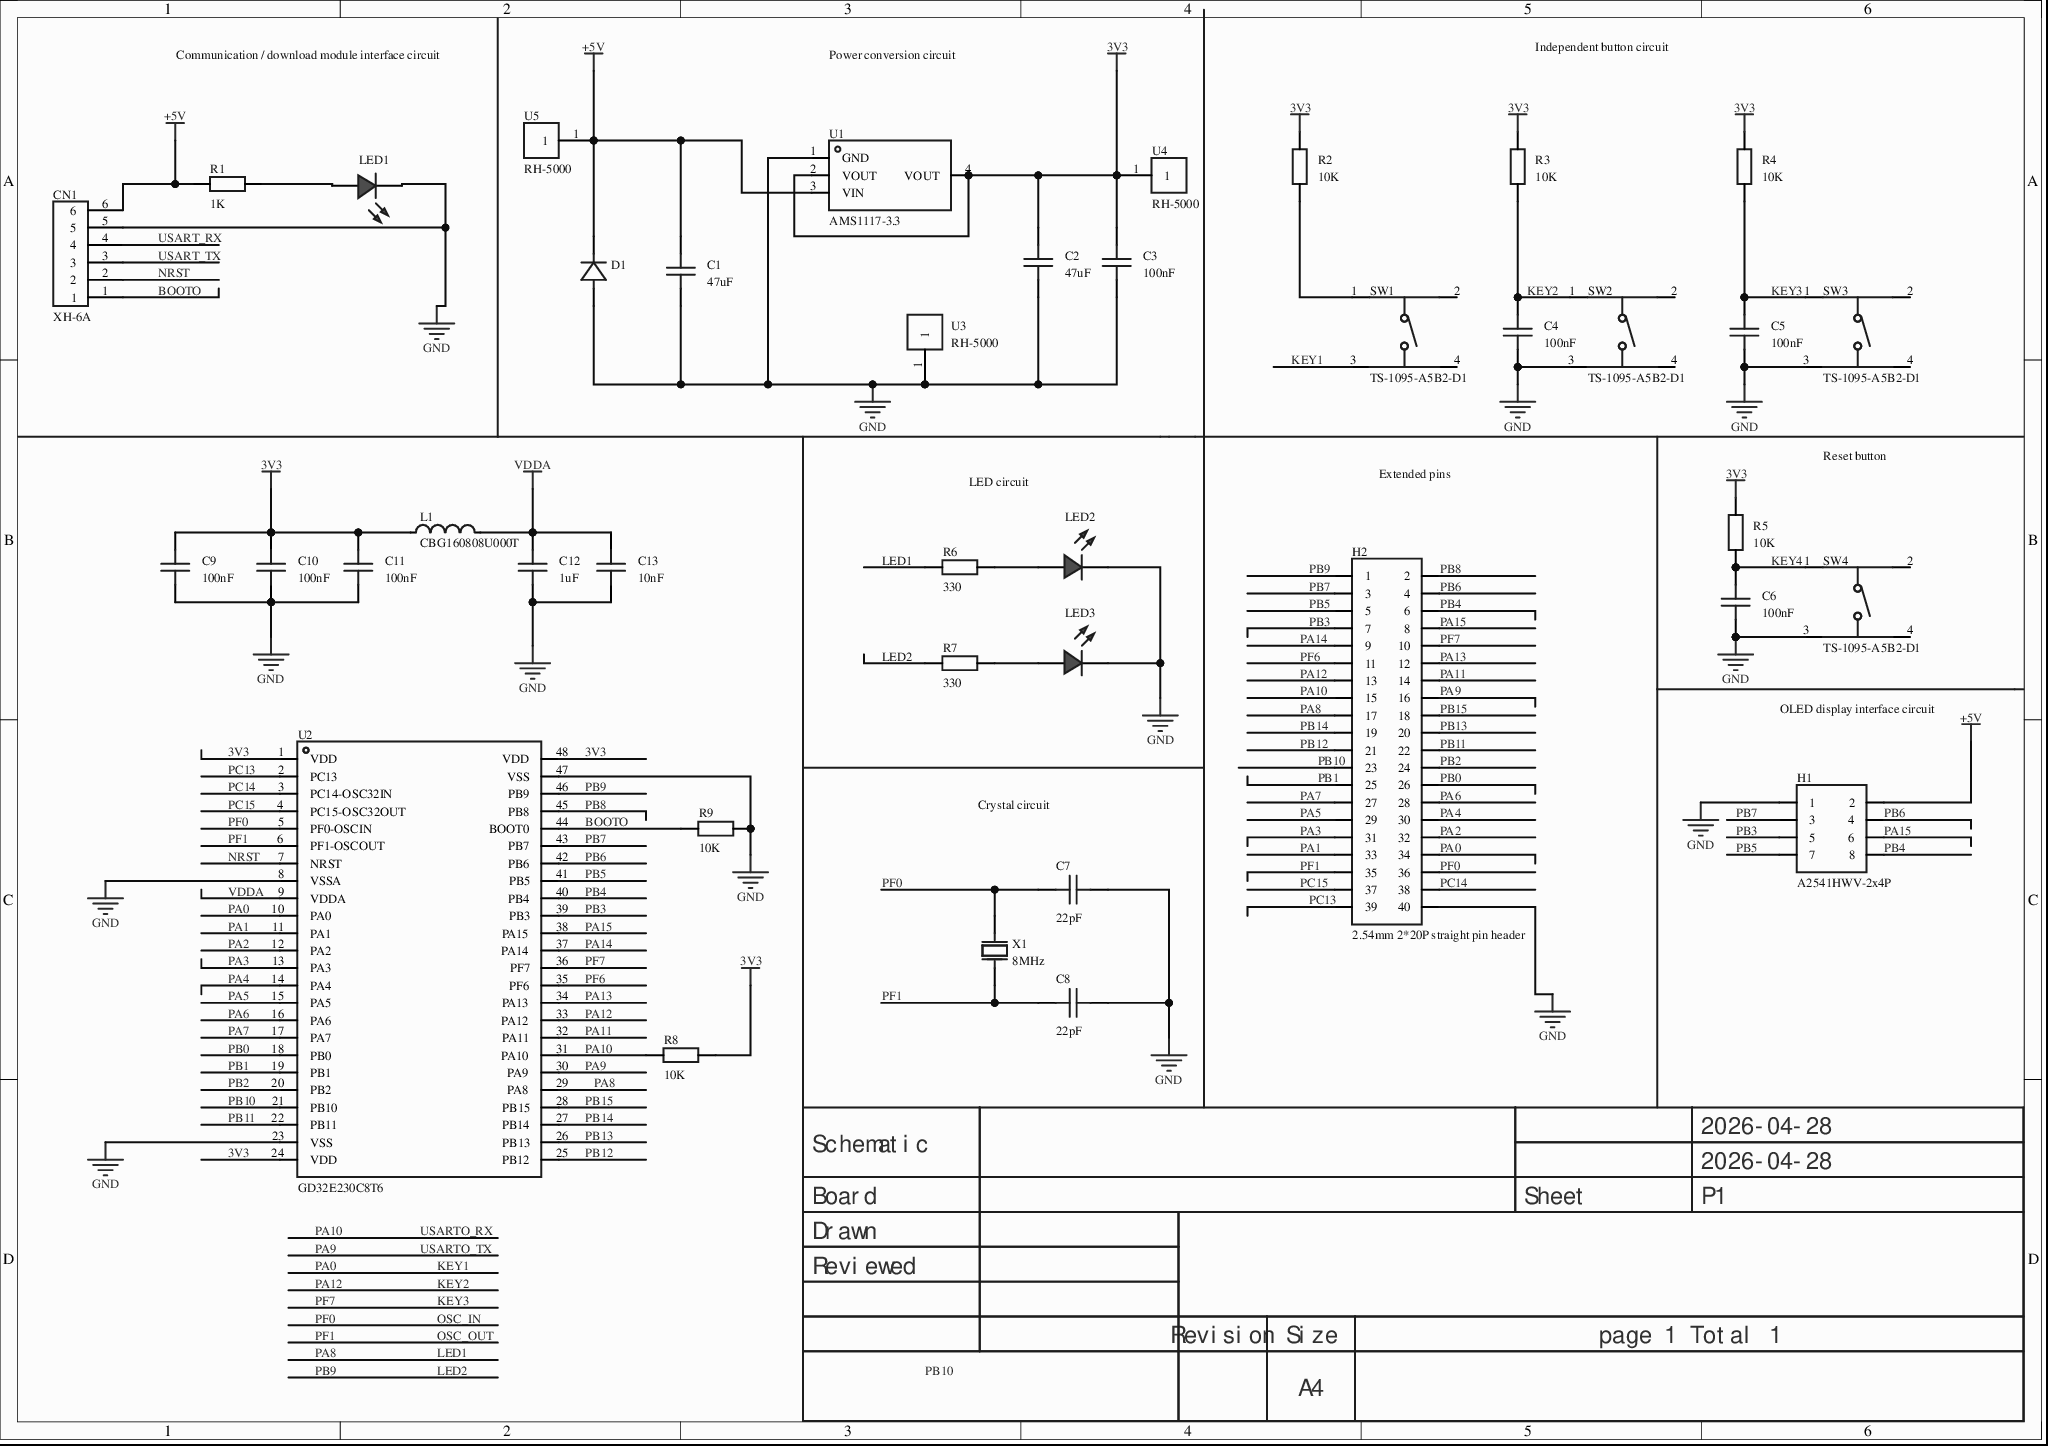
[diagram p0: MISC75379-3.schdoc]
# Altium project MISC75379-2.PrjPcb
1 sheet, 40 parts. Net scope: global (net labels, ports and power ports of the same name join across sheets).
Board file: MISC75379.pcbdoc

## Sheet MISC75379-3.schdoc
size 297 x 209 mm; Version: V1.0; @Project Name: MISC75379; @Update Date: 2026-04-28; @Create Date: 2026-04-28; @Board Name: MISC75379; @Create Time: 14:08:04; @Page Count: 1; @Page No: 1; @Schematic Name: MISC75379; @Update Time: 14:08:04; Size: A4

### Parts
C1  47uF  [C0603]
C2  47uF  [C0603]
C3  100nF  [C0603]
C4  100nF  [C0603]
C5  100nF  [C0603]
C6  100nF  [C0603]
C7  22pF  [C0603]
C8  22pF  [C0603]
C9  100nF  [C0603]
C10  100nF  [C0603]
C11  100nF  [C0603]
C12  1uF  [C0603]
C13  10nF  [C0603]
CN1  XH-6A  [CONN-TH_6P-P2.50_XH-6A]
D1  (no value)  [DO_1N4007]
H1  A2541HWV-2x4P  [HDR-TH_8P-P2.54-V-F-R2-C4-S2.54-1]
H2  2.54mm 2*20P straight pin header  [HDR-TH_40P-P2.54-V-M-R2-C20-S2.54]
L1  CBG160808U000T  [L0603]
LED1  (no value)  [LED_TH-3mm]
LED2  (no value)  [LED_TH-3mm]
LED3  (no value)  [LED_TH-3mm]
R1  1K  [R0603]
R2  10K  [R0603]
R3  10K  [R0603]
R4  10K  [R0603]
R5  10K  [R0603]
R6  330  [R0603]
R7  330  [R0603]
R8  10K  [R0603]
R9  10K  [R0603]
SW1  TS-1095-A5B2-D1  [SW-TH_4P-L6.0-W6.0-P4.50-LS6.5]
SW2  TS-1095-A5B2-D1  [SW-TH_4P-L6.0-W6.0-P4.50-LS6.5]
SW3  TS-1095-A5B2-D1  [SW-TH_4P-L6.0-W6.0-P4.50-LS6.5]
SW4  TS-1095-A5B2-D1  [SW-TH_4P-L6.0-W6.0-P4.50-LS6.5]
U1  AMS1117-3.3  [SOT-223-3_L6.5-W3.4-P2.30-LS7.0-BR]
U2  GD32E230C8T6  [LQFP-48_L7.0-W7.0-P0.50-LS9.0-BL]
U3  RH-5000  [TEST-TH_BD2.54-P1.4_RED]
U4  RH-5000  [TEST-TH_BD2.54-P1.4_RED]
U5  RH-5000  [TEST-TH_BD2.54-P1.4_RED]
X1  8MHz  [CRYSTAL-SMD_L11.5-W4.8-LS12.7]

### Nets
3V3: C2.2 C3.2 C9.2 C10.2 C11.2 L1.1 R2.2 R3.2 R4.2 R5.2 R8.2 U1.2(VOUT) U1.4(VOUT) U2.1(VDD) U2.24(VDD) U2.48(VDD) U4.1
+5V: C1.2 CN1.6 D1.1(K) H1.2 R1.1 U1.3(VIN) U5.1
GND: C1.1 C2.1 C3.1 C4.1 C5.1 C6.1 C7.2 C8.2 C9.1 C10.1 C11.1 C12.1 C13.1 CN1.5 D1.2(A) H1.1 H2.40 LED1.2(A) LED2.2(A) LED3.2(A) R9.2 SW2.3 SW3.3 SW4.3 U1.1(GND) U2.8(VSSA) U2.23(VSS) U2.47(VSS) U3.1
VDDA: C12.2 C13.2 L1.2 U2.9(VDDA)
BOOTO: CN1.1 R9.1 U2.44(BOOT0)
KEY1: H2.34 SW1.3 U2.10(PA0)  [also labelled PA0]
KEY2: C4.2 H2.13 R3.1 SW2.1 U2.33(PA12)  [also labelled PA12]
KEY3: C5.2 H2.10 R4.1 SW3.1 U2.36(PF7)  [also labelled PF7]
KEY4: C6.2 R5.1 SW4.1
LED1: H2.17 U2.29(PA8)  [also labelled PA8]
LED2: H2.1 U2.46(PB9)  [also labelled PB9]
NRST: CN1.2 U2.7(NRST)
OSC_IN: C7.1 H2.36 U2.5(PF0-OSCIN) X1.1(OSC1)  [also labelled PF0]
OSC_OUT: C8.1 H2.35 U2.6(PF1-OSCOUT) X1.2(OSC2)  [also labelled PF1]
PA1: H2.33 U2.11(PA1)
PA2: H2.32 U2.12(PA2)
PA3: H2.31 U2.13(PA3)
PA4: H2.30 U2.14(PA4)
PA5: H2.29 U2.15(PA5)
PA6: H2.28 U2.16(PA6)
PA7: H2.27 U2.17(PA7)
PA9: H2.16 U2.30(PA9)  [also labelled USARTO_TX]
PA10: H2.15 R8.1 U2.31(PA10)  [also labelled USARTO_RX]
PA11: H2.14 U2.32(PA11)
PA13: H2.12 U2.34(PA13)
PA14: H2.9 U2.37(PA14)
PA15: H1.6 H2.8 U2.38(PA15)
PB0: H2.26 U2.18(PB0)
PB1: H2.25 U2.19(PB1)
PB2: H2.24 U2.20(PB2)
PB3: H1.5 H2.7 U2.39(PB3)
PB4: H1.8 H2.6 U2.40(PB4)
PB5: H1.7 H2.5 U2.41(PB5)
PB6: H1.4 H2.4 U2.42(PB6)
PB7: H1.3 H2.3 U2.43(PB7)
PB8: H2.2 U2.45(PB8)
PB10: H2.23 U2.21(PB10)
PB11: H2.22 U2.22(PB11)
PB12: H2.21 U2.25(PB12)
PB13: H2.20 U2.26(PB13)
PB14: H2.19 U2.27(PB14)
PB15: H2.18 U2.28(PB15)
PC13: H2.39 U2.2(PC13)
PC14: H2.38 U2.3(PC14-OSC32IN)
PC15: H2.37 U2.4(PC15-OSC32OUT)
PF6: H2.11 U2.35(PF6)
USART_RX: CN1.4
USART_TX: CN1.3
NetLED1_1: LED1.1(C) R1.2
NetLED2_1: LED2.1(C) R6.2
NetLED3_1: LED3.1(C) R7.2
NetR2_1: R2.1 SW1.1

Not connected (* = marked no-connect by the designer): R6 1; R7 1; SW1 2 4; SW2 2 4; SW3 2 4; SW4 2 4

### Notes on the sheet
- Communication / download module interface circuit
- Power conversion circuit
- Independent button circuit
- LED circuit
- Extended pins
- Reset button
- (near R6) LED1
- (near R7) LED2
- OLED display interface circuit
- Crystal circuit
- Labels drawn without touching a wire or pin: PB10
- 2026-04-28
- Schematic
- Board
- Sheet
- P1
- Drawn
- Reviewed
- Revision
- Size
- A4
- page 1 Total 1

### Library data of the parts
C1 C2 = CAP_0603: Symbol: Capacitance; ConvertToPcb: yes; ModelId: ac125912035d415993ca9572d50418b10819f05c4eef4c71ace90d822a990e87; ModelName: C0603_L1.6-W0.8-H0.8; ModelTransform: 62.992,31.496,0,0,0,0,0,0,0; Value: 100nF; Device: CAP_0603; AddInBom: yes; Supplier Footprint: 0603; FootprintName: C0603
C3 = CAP_0603: Symbol: Capacitance; ConvertToPcb: yes; ModelId: ac125912035d415993ca9572d50418b10819f05c4eef4c71ace90d822a990e87; ModelName: C0603_L1.6-W0.8-H0.8; ModelTransform: 62.992,31.496,0,0,0,0,0,0,0; Device: CAP_0603; AddInBom: yes; Supplier Footprint: 0603; FootprintName: C0603; Value: 100nF
C4-C13 = CAP_0603: Symbol: Capacitance; 3D Model: ac125912035d415993ca9572d50418b10819f05c4eef4c71ace90d822a990e87; 3D Model Transform: 62.992,31.496,0,0,0,0,0,0,0; ConvertToPcb: yes; ModelName: C0603_L1.6-W0.8-H0.8; Device: CAP_0603; Supplier Footprint: 0603; AddInBom: yes; FootprintName: C0603
  C4-C6 C9-C11: Value: 100nF
  C7 C8: Value: 22pF
  C12: Value: 1uF
  C13: Value: 10nF
CN1 = XH-6A_C5663: Pin structure: 1x6P; pitch: 2.5mm; mounting: through-hole; reference series: XH; total PIN count: 6P; rows: 1; pins per row: 6; row pitch: -; rated current: -; contact material: -; contact plating: -; operating temperature: -;; Manufacturer: BOOMELE(博穆精密); AddInBom: yes; ModelId: 736bda21d9714549b61b9aaa09ca89560819f05c4eef4c71ace90d822a990e87; ModelName: XH2.5-6A; ModelTransform: 688.975,374.015,0,0,90,0,0,94.488,90.551; Number of PINs Per Row: 6; Z-Height of the Board: 7mm; X-Length of Bottom Edge on Board (Spacing Line): 17.5mm; Y-Width of Bottom Edge on Board: 5.8mm; Symbol: XH-6A; Device: XH-6A_C5663; LCSC Part Name: 1x6P 间距:2.5mm 直插 系列:XH; SupplierPart: C5663; ManufacturerPart: XH-6A; Supplier Footprint: 插件,P=2.5mm; JLCPCB Part Class: Extended Part; Datasheet: https://item.szlcsc.com/datasheet/XH-6A/6115.html; Supplier: LCSC; ConvertToPcb: yes; FootprintName: CONN-TH_6P-P2.50_XH-6A; Pins Structure: 1x6P; Pitch: 2.5mm; Mounting Type: Through-hole; Reference Series: XH; Number of Pins: 6P; Number of Rows: 1; Row Spacing: -; Current Rating: -; Contact Material: -; Contact Plating: -; Operating Temperature: -; Voltage Rating: -; Plastic Material: -; Flame Retardant Rating: -; Supplementary Features: -; Color: White
D1 = D_1N4007A: AddInBom: yes; ModelId: 6de1e9b71a0d4751b4e9df530304c1a30819f05c4eef4c71ace90d822a990e87; ModelName: DO-41_D2.4-L4.7-P8.70; ModelTransform: 373.9,94.4,232.29,0,0,0,0,0,-140; Symbol: D_1N4007; Device: D_1N4007A; Supplier Footprint: DO-41; ConvertToPcb: yes; FootprintName: DO_1N4007
H1 = A2541HWV-2x4P: Socket structure: 2x4P; pitch: 2.54mm; row pitch: 2.54mm; round/square hole: square hole; mounting: through-hole; rows: double row; total hole count: 8P; rated current: 3A; rated voltage: 250V; socket direction: top; plastic height: 8.5mm; contact material: brass; contact plating: gold; operating temperature: -40℃~+105℃;; Manufacturer: CJT(长江连接器); AddInBom: yes; ModelId: 64729f32a5874cf59655d275a66f10500819f05c4eef4c71ace90d822a990e87; ModelName: HDR2.54-F-LI-2X4P; ModelTransform: 399.999,200,0,0,0,0,0,0,-118.11; PIN Length: 3.2mm; Symbol: A2541HWV-2X4P; Device: A2541HWV-2x4P; LCSC Part Name: 2x4P 间距:2.54mm 直插; SupplierPart: C239344; ManufacturerPart: A2541HWV-2x4P; Supplier Footprint: 插件,P=2.54mm; JLCPCB Part Class: Extended Part; Datasheet: https://item.szlcsc.com/datasheet/A2541HWV-2x4P/238448.html; Supplier: LCSC; ConvertToPcb: yes; FootprintName: HDR-TH_8P-P2.54-V-F-R2-C4-S2.54-1; Holes Structure: 2x4P; Pitch: 2.54mm; Row Spacing: 2.54mm; Circular Hole / Square Hole: Square hole; Mounting Type: Through-hole; Number of Rows: Double row; Number of Positions: 8P; Current Rating: 3A; Voltage Rating (Max): 250V; Holes Direction: Top; Insulation Height: 8.5mm; Contact Material: Brass; Contact Plating: Gold; Operating Temperature: -40℃~+105℃
H2 = 2.54mm 2*20P直排针: Pin structure: 2x20P; pitch: 2.54mm; row pitch: 2.54mm; round/square pin: square pin; mounting: through-hole; rows: double row; total PIN count: 40P; rated current: 3A; rated voltage: -; mating pin length: 6mm; plastic height: -; tail length: 3mm; contact material: brass; contact plating: -; operating temperature: -40℃~+105℃; color: black;; Manufacturer: BOOMELE(博穆精密); Symbol: Header-Male-2.54_2x20; AddInBom: yes; ModelId: 2f697d2f705a4509bdac70452e51b3cc0819f05c4eef4c71ace90d822a990e87; ModelName: HDR-TH_40P-P2.54-M-LI-2X20P; ModelTransform: 1999.996,196.85,0,0,0,0,0,0,-118.11; Device: 2.54mm 2*20P straight pin header; LCSC Part Name: 2x20P 间距:2.54mm 方针 直插; SupplierPart: C50980; ManufacturerPart: 2.54mm 2*20P直排针; Supplier Footprint: 插件,P=2.54mm; JLCPCB Part Class: Extended Part; Datasheet: https://item.szlcsc.com/datasheet/2.54mm%25202*20P%25E7%259B%25B4%25E6%258E%2592%25E9%2592%2588/51992.html; Supplier: LCSC; ConvertToPcb: yes; FootprintName: HDR-TH_40P-P2.54-V-M-R2-C20-S2.54; Pin Structure: 2x20P; Pitch: 2.54mm; Row Spacing: 2.54mm; Circluar Pins/Square Pins: Square pin; Mounting Type: Through-hole; Number of Rows: Double row; Number of Pins: 40P; Current Rating: 3A; Voltage Rating (Max): -; Length of Mating Pin: 6mm; Insulation Height: -; Length of End Connection Pin: 3mm; Contact Material: Brass; Contact Plating: -; Operating Temperature: -40℃~+105℃; Color: Black
L1 = CBG160808U000T: Impedance@frequency: 0Ω@100MHz; DC resistance (DCR): 100mΩ;; Manufacturer: FH(风华); AddInBom: yes; ModelId: 2bc5ec593d464d6ba9807aec0b5673c20819f05c4eef4c71ace90d822a990e87; ModelName: L0603_L1.6-W0.8-H0.5_BEAD; ModelTransform: 62.992,31.496,0,180,0,0,0.094,0.629,0; Current Rating: 800mA; Number of Circuits: 1; Symbol: CBG160808U000T; Device: CBG160808U000T; LCSC Part Name: 单路 0603磁珠 阻抗0Ω@100MHz; SupplierPart: C43163; ManufacturerPart: CBG160808U000T; Supplier Footprint: 0603; JLCPCB Part Class: Extended Part; Datasheet: https://item.szlcsc.com/datasheet/CBG160808U000T/44154.html; Supplier: LCSC; ConvertToPcb: yes; FootprintName: L0603; Impedance @ Frequency: 0Ω@100MHz; DC Resistance(DCR): 100mΩ; Operating Temperature: -40℃~+85℃
LED1-LED3 = LED_TH-R_3mm: 3D Model: a497c992633541038a38947cdc58012f0819f05c4eef4c71ace90d822a990e87; 3D Model Transform: 141.274,153.327,0,0,0,0,-5.984,0,-137.795; ConvertToPcb: yes; ModelName: LED-TH-3mm_R; Symbol: LED_TH-R; Device: LED_TH-R_3mm; Supplier Footprint: 插件; AddInBom: yes; FootprintName: LED_TH-3mm
R1 = Res_0603: Symbol: Resistor; 3D Model: fc143cca1e79419f9cd78b61e9279f080819f05c4eef4c71ace90d822a990e87; 3D Model Transform: 31.8897,63.7794,0,90,0,0,0,0,0; Value: 10K; ConvertToPcb: yes; Device: Res_0603; Supplier Footprint: 0603; AddInBom: yes; FootprintName: R0603; ModelName: R0603
R2-R9 = Res_0603: Symbol: Resistor; 3D Model: fc143cca1e79419f9cd78b61e9279f080819f05c4eef4c71ace90d822a990e87; 3D Model Transform: 31.8897,63.7794,0,90,0,0,0,0,0; ConvertToPcb: yes; Device: Res_0603; Supplier Footprint: 0603; AddInBom: yes; FootprintName: R0603; ModelName: R0603
  R2-R5 R8 R9: Value: 10K
  R6 R7: Value: 330
SW1-SW4 = TS-1095-A5B2-D1: Circuit structure: SPST; button shape: round button; actuating force: 180gf; mounting: through-hole; switch length: 6mm; switch width: 6mm; switch height: 6mm; bracket: none; mechanical life: -;; Manufacturer: Yuandi(元迪); AddInBom: yes; ModelId: 20eee248bc684ccd8cbdbb1d0d91ec6f0819f05c4eef4c71ace90d822a990e87; ModelName: SW-TH_4P-L6.0-W6.0-H5.0-LS6.5-P4.50; ModelTransform: 236.22,323.03,0,90,0,0,0,0,-137.795; Actuator/Cap Color: Black; Pin Style: PC pin; Symbol: TS-1095-A5B2-D1; Device: TS-1095-A5B2-D1; LCSC Part Name: 6*6*6mm 直插 轻触开关; SupplierPart: C782808; ManufacturerPart: TS-1095-A5B2-D1; Supplier Footprint: 插件; JLCPCB Part Class: Extended Part; Datasheet: https://atta.szlcsc.com/upload/public/pdf/source/20200908/C782804_D14F61DCCBE05C7EE913124CF28857B3.pdf; Supplier: LCSC; ConvertToPcb: yes; FootprintName: SW-TH_4P-L6.0-W6.0-P4.50-LS6.5; Circuit: SPST; Actuator Style: Round button; Operating Force: 180gf; Mounting Style: Through-hole; Switch Length: 6mm; Switch Width: 6mm; Switch Height: 6mm; Strike Gundam: None; Mechanical Life: -
U1 = AMS1117-3.3_C6186: Output type: fixed; working voltage: 15V; output voltage: 3.3V; output current: 1A; ripple rejection (PSRR): 72dB@(120Hz); output polarity: positive;; Manufacturer: AMS; AddInBom: yes; ModelId: 925194bf9823436183a3e0b978a8d0760819f05c4eef4c71ace90d822a990e87; ModelName: SOT-223-4P_L6.5-W3.5-H1.6-LS7.0-P2.30; ModelTransform: 279.89794,255.905,0,180,0,0,-3.9385,-0.0005,0; Voltage Dropout: 1.1V@(800mA); standby current: 5mA; Noise: 0.003%Vout; Number of Outputs: 1; Symbol: AMS1117-3.3; Device: AMS1117-3.3_C6186; LCSC Part Name: 3.3V 1A 15V; SupplierPart: C6186; ManufacturerPart: AMS1117-3.3; Supplier Footprint: SOT-223; JLCPCB Part Class: Basic Part; Datasheet: https://item.szlcsc.com/datasheet/AMS1117-3.3/6652.html; Supplier: LCSC; ConvertToPcb: yes; FootprintName: SOT-223-3_L6.5-W3.4-P2.30-LS7.0-BR; Output Type: Fixed; Voltage - Supply: 15V; Output Voltage: 3.3V; Output Current: 1A; Power Supply Rejection Ratio (PSRR): 72dB@(120Hz); Features: Overcurrent protection; thermal shutdown; Operating Temperature: -40℃~+125℃; Output Configuration: Positive
U2 = GD32E230C8T6: CPU core: ARM-M series; max CPU frequency: 72MHz; application field: -;; Manufacturer: GigaDevice(兆易创新); AddInBom: yes; ModelId: 093be70396ff421eb2cdb946d5311efc0819f05c4eef4c71ace90d822a990e87; ModelName: LQFP-48_L7.0-W7.0-H1.4-LS9.0-P0.50; ModelTransform: 354.331,354.331,0,0,0,0,0,0,0; Program Storage Size: 64KB; Program Memory Type: FLASH; Number of I/O: 39; ADC (Bit): 12bit; PWM (Bit): 16bit; Voltage - Supply: 1.8V~3.6V; Symbol: GD32E230C8T6; Device: GD32E230C8T6; LCSC Part Name: ARM Cortex-M23 32位微控制器（MCU）; SupplierPart: C380535; ManufacturerPart: GD32E230C8T6; Supplier Footprint: LQFP-48(7x7); JLCPCB Part Class: Extended Part; Datasheet: https://item.szlcsc.com/datasheet/GD32E230C8T6/352855.html; Supplier: LCSC; ConvertToPcb: yes; FootprintName: LQFP-48_L7.0-W7.0-P0.50-LS9.0-BL; CPU Core: ARM-M series; CPU Maximum Speed: 72MHz; Applications: -
U3-U5 = RH-5000: Manufacturer: 荣和; AddInBom: yes; ModelId: 3ee70e2a8afb47659abb73033ae4c5d50819f05c4eef4c71ace90d822a990e87; ModelTransform: 98.425,98.79098,0,0,0,0,0,0,-125.984; Connector Type: Pin type (through-board); Plastic Color: Red; Board Space (Diameter φ/ Length x Width): 2.5mm; Symbol: RH-5000; Device: RH-5000; LCSC Part Name: PCB电路板测试点/测试针; SupplierPart: C5277086; ManufacturerPart: RH-5000; Supplier Footprint: -; JLCPCB Part Class: Extended Part; Datasheet: https://item.szlcsc.com/datasheet/RH-5000/6009931.html; Supplier: LCSC; ConvertToPcb: yes; FootprintName: TEST-TH_BD2.54-P1.4_RED; ModelName: TEST-TH_BD2.54-P1.4_RED
X1 = X49SM8MSD2SC: Crystal type: SMD crystal; frequency: 8MHz; frequency tolerance at room temperature: ±20ppm; load capacitance: 20pF; frequency stability: ±30ppm;; Manufacturer: YXC(扬兴晶振); AddInBom: yes; ModelId: 6f569b91267b44029b8615eb5c810fba0819f05c4eef4c71ace90d822a990e87; ModelName: HC-49S_L11.4-W1.8-H3.0-LS12.7; ModelTransform: 499.999,188.976,0,180,0,0,0.002,-0.002,0; Symbol: X49SM8MSD2SC; Device: X49SM8MSD2SC; LCSC Part Name: HC-49SMD 8MHZ 20PF ±20PPM -20~70℃（±30PPM）; SupplierPart: C12674; ManufacturerPart: X49SM8MSD2SC; Supplier Footprint: HC-49S-SMD; JLCPCB Part Class: Basic Part; Datasheet: https://item.szlcsc.com/datasheet/X49SM8MSD2SC/13310.html; Supplier: LCSC; ConvertToPcb: yes; FootprintName: CRYSTAL-SMD_L11.5-W4.8-LS12.7; Type: SMD crystal; Value: 8MHz; Normal temperature Frequency Tolerance: ±20ppm; Load Capacitance: 20pF; Frequency Stability: ±30ppm; Operating Temperature: -20℃~+70℃